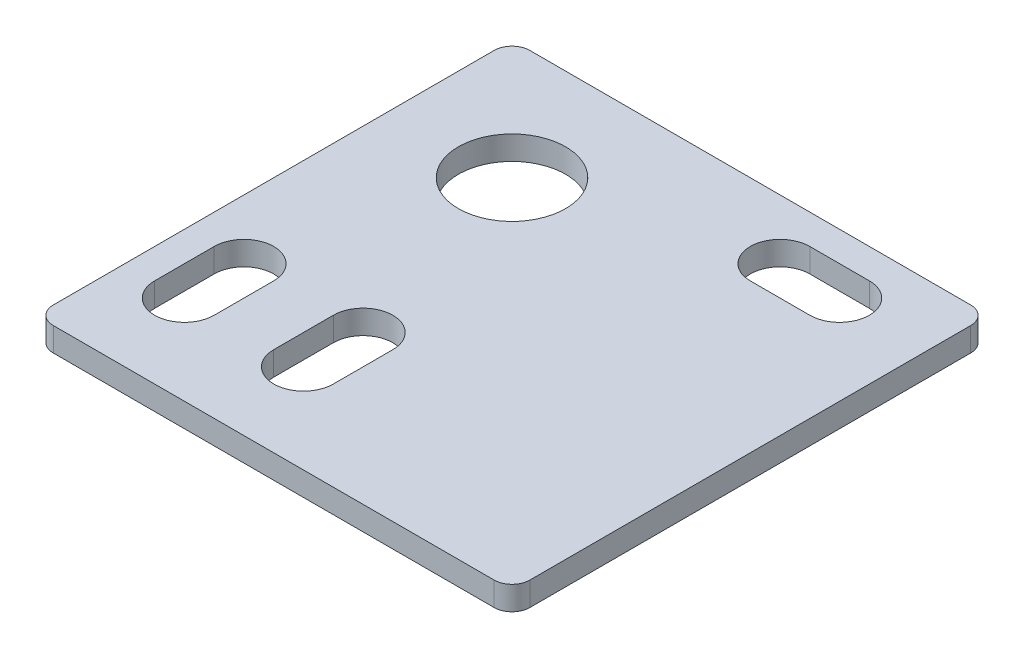
SolidWorks part; units mm, degrees
material "Q235"
ref_plane "Front" through (0, 0, 0) normal (0, 0, 1) x (1, 0, 0)
ref_plane "Top" through (0, 0, 0) normal (0, 1, 0) x (1, 0, 0)
ref_plane "Right" through (0, 0, 0) normal (1, 0, 0) x (0, 0, -1)
sketch "Sketch1" plane through (0, 0, 0) normal (0, 1, 0) x (1, 0, 0)
  line L0 (0, 0) -> (-80, 0)
  line L1 (-80, 0) -> (-80, -80)
  line L3 (-80, -80) -> (0, -80)
  line L4 (0, -80) -> (0, 0)
  line L5 (-25, -10) -> (-15, -10) construction
  line L6 (-25, -5) -> (-15, -5)
  line L7 (-25, -15) -> (-15, -15)
  line L8 (-70, -55) -> (-70, -65) construction
  line L9 (-65, -55) -> (-65, -65)
  line L10 (-75, -55) -> (-75, -65)
  line L11 (-50, -55) -> (-50, -65) construction
  line L12 (-45, -55) -> (-45, -65)
  line L13 (-55, -55) -> (-55, -65)
  circle A0 centre (-60, -20) radius 9
  arc A1 (-25, -5) -> (-25, -15) centre (-25, -10) ccw
  arc A2 (-15, -15) -> (-15, -5) centre (-15, -10) ccw
  arc A3 (-65, -55) -> (-75, -55) centre (-70, -55) ccw
  arc A4 (-75, -65) -> (-65, -65) centre (-70, -65) ccw
  arc A5 (-45, -55) -> (-55, -55) centre (-50, -55) ccw
  arc A6 (-55, -65) -> (-45, -65) centre (-50, -65) ccw
  point P10 (-20, -10)
  point P17 (-70, -60)
  point P22 (-50, -60)
  dimension "D5" = 18
  dimension "D11" = 60
  dimension "D7" = 60
  dimension "D1" = 80
  dimension "D2" = 80
  dimension "D3" = 20
  dimension "D4" = 20
  dimension "D6" = 10
  dimension "D8" = 10
  dimension "D9" = 10
  dimension "D12" = 10
  dimension "D13" = 10
  dimension "D14" = 10
  dimension "D15" = 50
  dimension "D16" = 20
extrude "Boss-Extrude1" add sketch "Sketch1" along normal blind 4
fillet "Fillet1" radius 3 4 edges at (0, 2, 80) (-80, 2, 80) (0, 2, 0) (-80, 2, 0)
